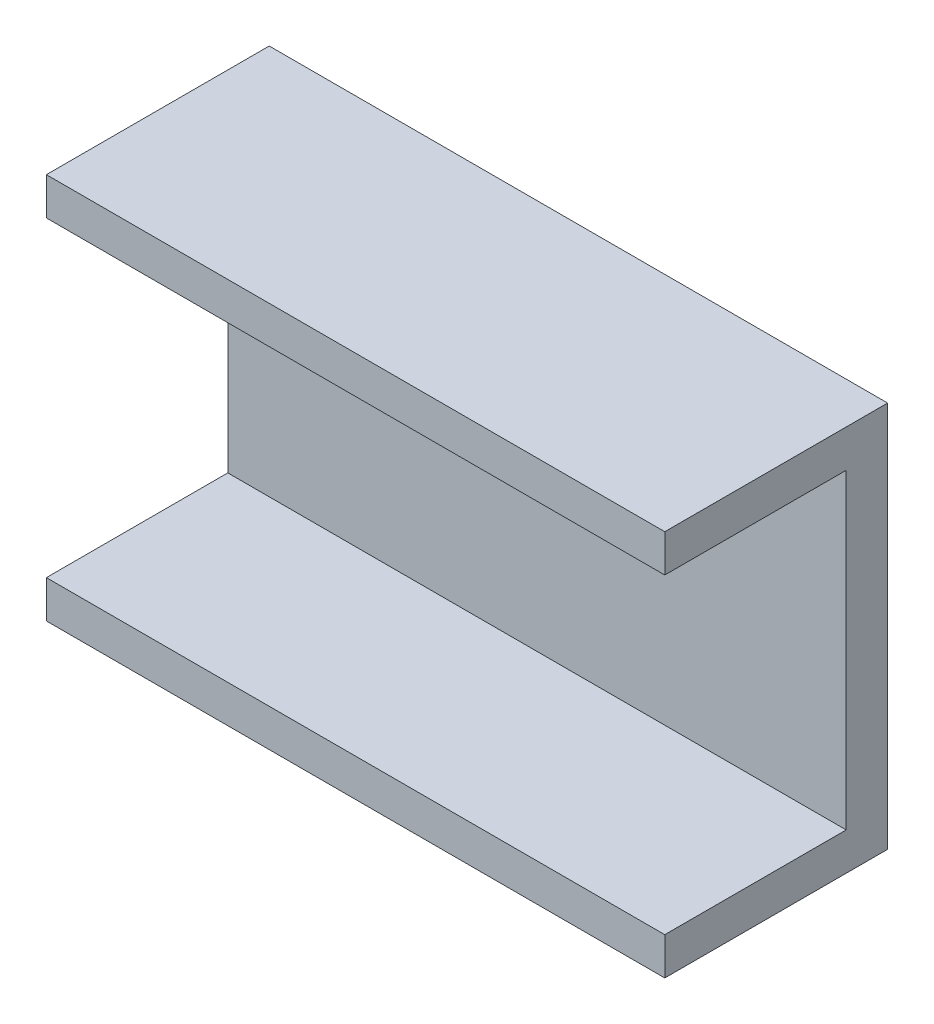
from build123d import *

# Parameters (mm, degrees)
SKETCH1_W           = 80
SKETCH1_H           = 50
BOSS_EXTRUDE1_DEPTH = 28.83
SKETCH2_W           = 23.467762578
SKETCH2_H           = 40.294008895
CUT_EXTRUDE1_DEPTH  = 99.646687223


with BuildPart() as part:
    # Sketch1 → Boss-Extrude1 (new body)
    with BuildSketch(Plane.XY):
        with Locations((40, 25)):
            Rectangle(SKETCH1_W, SKETCH1_H)
    extrude(amount=BOSS_EXTRUDE1_DEPTH)

    # Sketch2 → Cut-Extrude1 (cut, through all)
    with BuildSketch(Plane(origin=(80, 0, 0), x_dir=(0, 0, -1), z_dir=(1, 0, 0))):
        with Locations((-17.096118711, 25.002275375)):
            Rectangle(SKETCH2_W, SKETCH2_H)
    extrude(amount=-CUT_EXTRUDE1_DEPTH, mode=Mode.SUBTRACT)


solid = part.part
